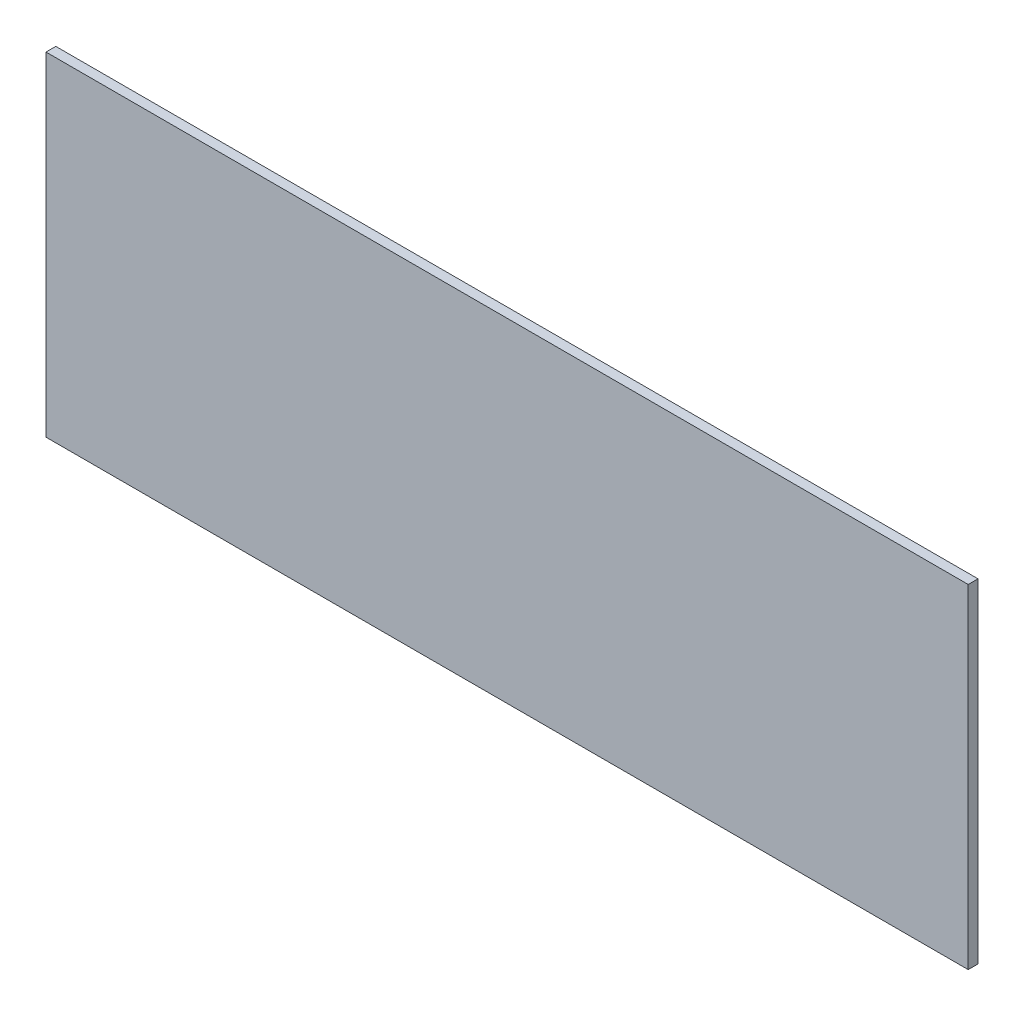
from build123d import *

# Parameters (mm, degrees)
SKETCH_1_W      = 470
SKETCH_1_H      = 170
EXTRUDE_1_DEPTH = 5


with BuildPart() as part:
    # 草图1 → 凸台-拉伸1 (new body)
    with BuildSketch(Plane.XY):
        with Locations((235, 85)):
            Rectangle(SKETCH_1_W, SKETCH_1_H)
    extrude(amount=EXTRUDE_1_DEPTH)


solid = part.part
